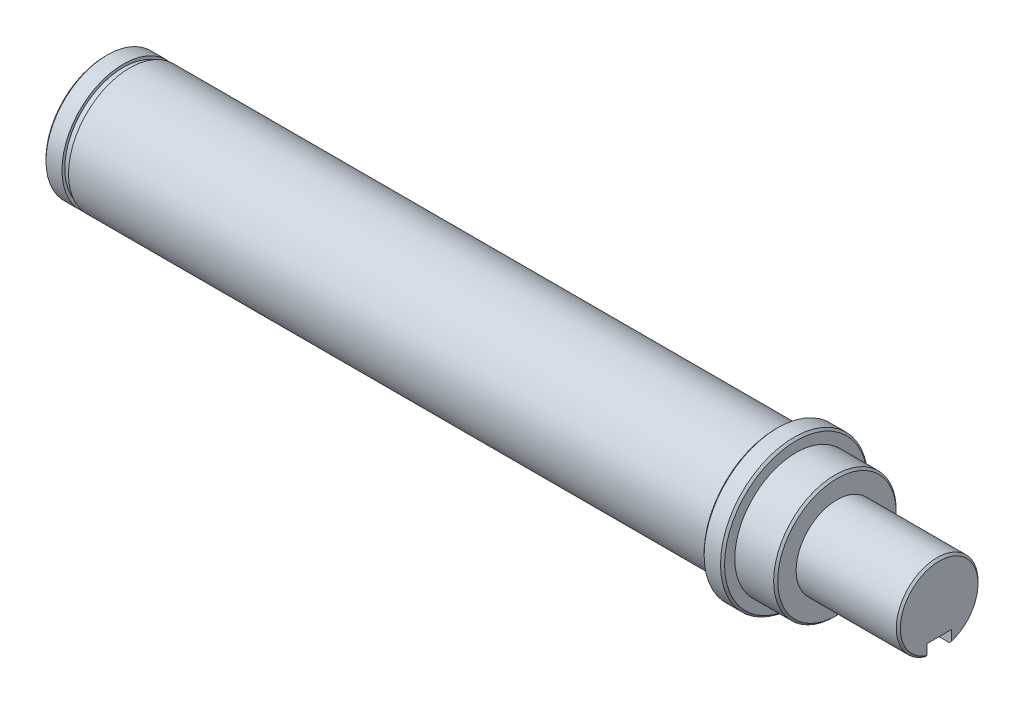
from build123d import *

# Parameters (mm, degrees)
CHAMFER_1_SIZE      = 0.5
CUT_EXTRUDE_1_DEPTH = 4
CUT_EXTRUDE_2_DEPTH = 3.5


with BuildPart() as part:
    # 草图1 → 旋转1 (revolve)
    with BuildSketch(Plane.XY, mode=Mode.PRIVATE) as revolve_1_sk:
        Polygon((0, 0), (0, 15), (4.4, 15), (4.4, 14.3), (6, 14.3), (6, 15), (164, 15), (164, 18), (169, 18), (169, 15), (179, 15), (179, 10), (204, 10), (204, 0), align=None)
    revolve(revolve_1_sk.sketch.rotate(Axis((0, 0, 0), (1, 0, 0)), 90), axis=Axis((0, 0, 0), (1, 0, 0)))

    # 倒角1
    chamfer_1_edges = [part.edges().sort_by_distance(p)[0] for p in [
        (204, 0, -10),
        (179, 0, -15),
        (169, 0, -18),
        (164, 0, -18),
        (0, 0, -15),
    ]]
    chamfer(chamfer_1_edges, length=CHAMFER_1_SIZE)

    # 草图2 → 切除-拉伸1 (cut)
    with BuildSketch(Plane(origin=(0, -15, 0), x_dir=(-1, 0, 0), z_dir=(0, -1, 0))):
        with BuildLine():
            Line((-49, -4), (-119, -4))
            ThreePointArc((-119, -4), (-123, 0), (-119, 4))
            Line((-119, 4), (-49, 4))
            ThreePointArc((-49, 4), (-45, 0), (-49, -4))
        make_face()
    extrude(amount=-CUT_EXTRUDE_1_DEPTH, mode=Mode.SUBTRACT)

    # 草图3 → 切除-拉伸2 (cut)
    with BuildSketch(Plane(origin=(0, -10, 0), x_dir=(-1, 0, 0), z_dir=(0, -1, 0))):
        with BuildLine():
            Line((-204, 3), (-184, 3))
            ThreePointArc((-184, 3), (-181, 0), (-184, -3))
            Line((-184, -3), (-204, -3))
            ThreePointArc((-204, -3), (-207, 0), (-204, 3))
        make_face()
    extrude(amount=-CUT_EXTRUDE_2_DEPTH, mode=Mode.SUBTRACT)


solid = part.part
